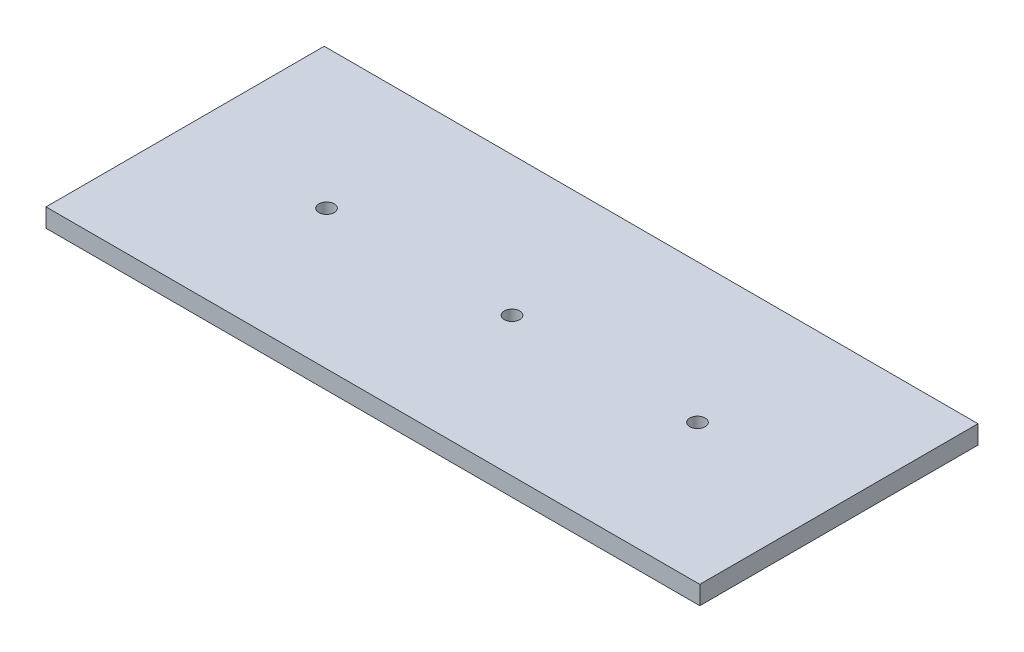
SolidWorks part; units mm, degrees
material "A3"
ref_plane "Front Plane" through (0, 0, 0) normal (0, 0, 1) x (1, 0, 0)
ref_plane "Top Plane" through (0, 0, 0) normal (0, 1, 0) x (1, 0, 0)
ref_plane "Right Plane" through (0, 0, 0) normal (1, 0, 0) x (0, 0, -1)
sketch "Sketch1" plane through (0, 0, 0) normal (0, 1, 0) x (1, 0, 0)
  line L1 (-70.5, 30) -> (70.5, 30)
  line L2 (-70.5, 30) -> (-70.5, -30)
  line L3 (-70.5, -30) -> (70.5, -30)
  line L4 (70.5, 30) -> (70.5, -30)
  line L5 (-70.5, 30) -> (70.5, -30) construction
  line L6 (-70.5, -30) -> (70.5, 30) construction
  point P0 (0, 0)
  dimension "D1" = 141
  dimension "D2" = 60
extrude "Boss-Extrude1" add sketch "Sketch1" along normal blind 4
hole_wizard "M4 Tapped Hole1" positions "Sketch3" profile "Sketch2" tap size "M4" standard "ISO" end condition through all
sketch "Sketch3" plane through (0, 4, 0) normal (0, 1, 0) x (1, 0, 0)
  line L1 (70.5, 30) -> (-70.5, 30) construction
  point P0 (-40, 0)
  point P2 (0, 0)
  point P4 (40, 0)
  dimension "D1" = 80
  dimension "D2" = 40
  dimension "D3" = 30
sketch "Sketch2" plane through (-40, 4, 0) normal (1, 0, 0) x (0, 0, 1)
  line L0 (0, 0) -> (0, 4)
  line L1 (0, 4) -> (1.65, 4)
  line L2 (1.65, 4) -> (1.65, 0)
  line L5 (1.65, 0) -> (0, 0)
  line L11 (0, -6.35) -> (0, 107.95) construction
  dimension "通孔螺纹孔钻头直径" = 3.3
  dimension "通孔螺纹孔钻头深度" = 4
cosmetic thread "Hole-Thread1"
cosmetic thread "Hole-Thread2"
cosmetic thread "Hole-Thread3"
